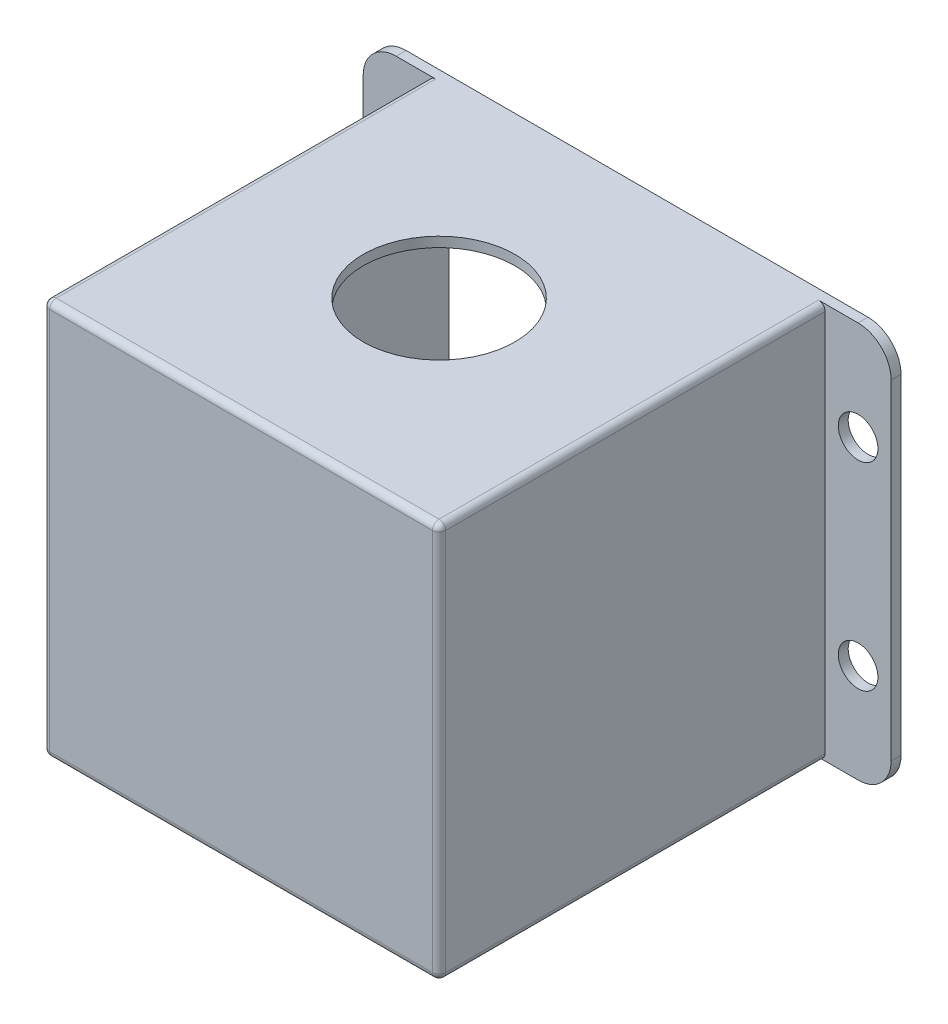
SolidWorks part; units mm, degrees
material "6061"
ref_plane "前视基准面" through (0, 0, 0) normal (0, 0, 1) x (1, 0, 0)
ref_plane "上视基准面" through (0, 0, 0) normal (0, 1, 0) x (1, 0, 0)
ref_plane "右视基准面" through (0, 0, 0) normal (1, 0, 0) x (0, 0, -1)
sketch "草图1" plane through (0, 0, 0) normal (0, 0, 1) x (1, 0, 0)
  line L1 (-30, 30) -> (30, 30)
  line L2 (-30, 30) -> (-30, -30)
  line L3 (-30, -30) -> (30, -30)
  line L4 (30, 30) -> (30, -30)
  line L5 (-30, 30) -> (30, -30) construction
  line L6 (-30, -30) -> (30, 30) construction
  point P0 (0, 0)
  dimension "D1" = 60
  dimension "D2" = 60
extrude "凸台-拉伸1" add sketch "草图1" along normal mid plane 60
shell "抽壳1" thickness 1.5
sketch "草图5" plane through (30, 0, 0) normal (1, 0, 0) x (0, 0, -1)
  line L0 (-30, 30) -> (30, 30) construction
  line L1 (30, -30) -> (28.5, -30)
  line L2 (30, -30) -> (30, 30)
  line L3 (30, 30) -> (28.5, 30)
  line L4 (28.5, -30) -> (28.5, 30)
  dimension "D1" = 1.5
extrude "凸台-拉伸3" add sketch "草图5" along normal blind 10
sketch "草图6" plane through (-30, 0, 0) normal (-1, 0, 0) x (0, 0, 1)
  line L0 (30, -30) -> (-30, -30) construction
  line L1 (-30, 30) -> (-28.5, 30)
  line L2 (-30, 30) -> (-30, -30)
  line L3 (-30, -30) -> (-28.5, -30)
  line L4 (-28.5, 30) -> (-28.5, -30)
  dimension "D1" = 1.5
extrude "凸台-拉伸4" add sketch "草图6" along normal blind 10
sketch "草图7" plane through (0, -30, 0) normal (0, -1, 0) x (1, 0, 0)
  line L0 (-40, -30) -> (40, -30) construction
  line L1 (-10, -15) -> (10, -15)
  line L2 (-10, -15) -> (-10, -30)
  line L3 (-10, -30) -> (10, -30)
  line L4 (10, -15) -> (10, -30)
  line L5 (0, 30) -> (0, -94.0306) construction
  line L6 (-30, 30) -> (30, 30) construction
  dimension "D1" = 20
  dimension "D2" = 15
extrude "切除-拉伸3" cut sketch "草图7" against normal up to next
fillet "圆角1" radius 5 2 edges at (10, -29.25, -15) (-10, -29.25, -15)
fillet "圆角2" radius 5 4 edges at (40, -30, -29.25) (-40, -30, -29.25) (-40, 30, -29.25) (40, 30, -29.25)
sketch "草图8" plane through (0, 30, 0) normal (0, 1, 0) x (1, 0, 0)
  circle A0 centre (0, 0) radius 11.5
  dimension "D1" = 23
extrude "切除-拉伸4" cut sketch "草图8" against normal up to next
fillet "圆角3" radius 1 8 edges at (30, 30, 0.75) (-30, 30, 0.75) (30, -30, 0.75) (-30, -30, 0.75) (30, 0, 30) (-30, 0, 30) (0, -30, 30) (0, 30, 30)
sketch "草图9" plane through (0, 0, -28.5) normal (0, 0, 1) x (1, 0, 0)
  line L0 (35, -30) -> (35, 30) construction
  line L1 (35, -30) -> (29, -30) construction
  line L2 (40, 25) -> (40, -25) construction
  line L6 (40, 0) -> (-40, 0) construction
  line L7 (-40, -25) -> (-40, 25) construction
  line L8 (0, -30) -> (0, 33.72) construction
  circle A0 centre (35, -15) radius 3
  circle A1 centre (35, 15) radius 3
  dimension "D3" = 6
  dimension "D2" = 30
  dimension "D1" = 5
extrude "切除-拉伸5" cut sketch "草图9" against normal through all
mirror "镜向1" about plane through (0, 0, 0) normal (1, 0, 0) of "切除-拉伸5"
